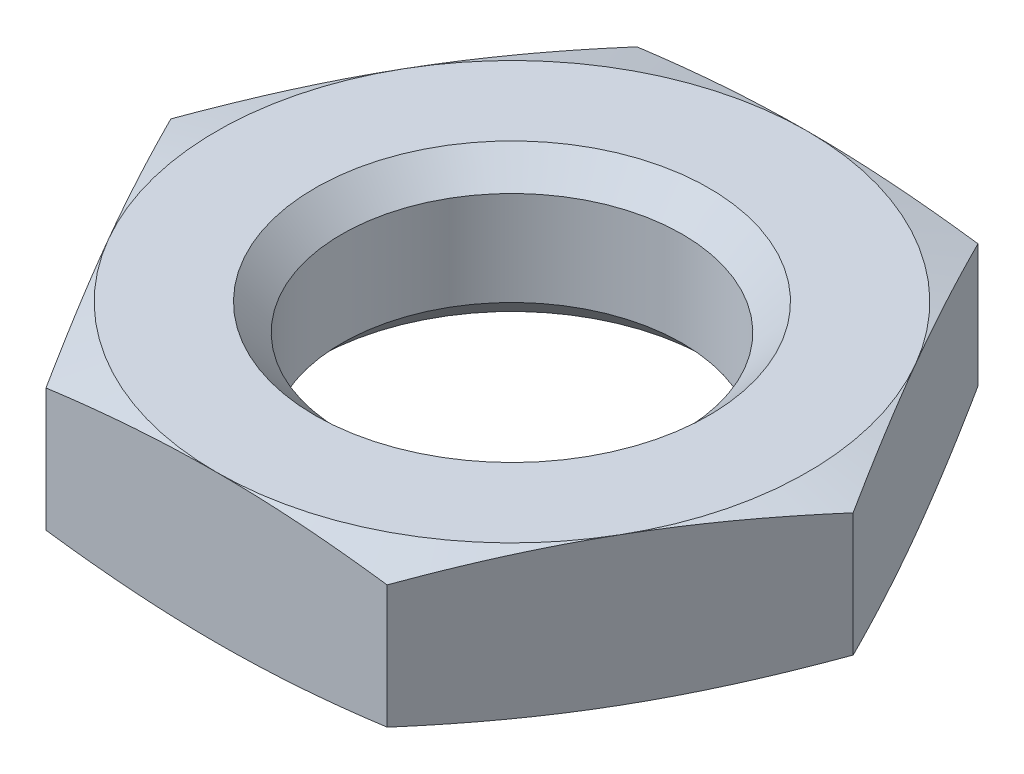
from build123d import *

# Parameters (mm, degrees)
CUT_EXTRUDE_1_DEPTH      = 1.5
CUT_EXTRUDE_1_DEPTH_BACK = 1.5
SKETCH_2_R               = 12


with BuildPart() as part:
    # 草图1 → 旋转1 (revolve)
    with BuildSketch(Plane.XY, mode=Mode.PRIVATE) as revolve_1_sk:
        Polygon((3.4585, -0.9585), (4, -1.5), (6, -1.5), (9.6, -0.535382907), (9.6, 0.535382907), (6, 1.5), (4, 1.5), (3.4585, 0.9585), align=None)
    revolve(revolve_1_sk.sketch.rotate(Axis((0, -1.5, 0), (0, 1, 0)), 270), axis=Axis((0, -1.5, 0), (0, 1, 0)))

    # 草图2 → 切除-拉伸1 (cut, two sides: drawn at the far end of the back side and taken through both)
    with BuildSketch(Plane(origin=(0, 0, 0), x_dir=(1, 0, 0), z_dir=(0, 1, 0)).offset(-CUT_EXTRUDE_1_DEPTH_BACK)):
        Circle(SKETCH_2_R)
        Polygon((-6.92820323, 0), (-3.464101615, -6), (3.464101615, -6), (6.92820323, 0), (3.464101615, 6), (-3.464101615, 6), align=None, mode=Mode.SUBTRACT)
    extrude(amount=CUT_EXTRUDE_1_DEPTH + CUT_EXTRUDE_1_DEPTH_BACK, mode=Mode.SUBTRACT)


solid = part.part
